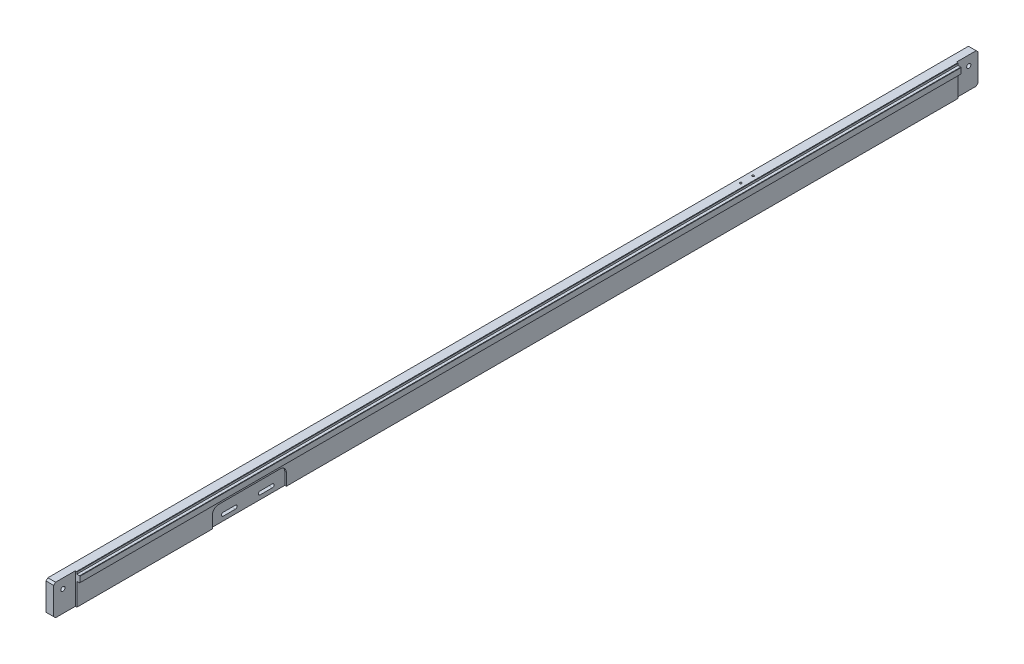
SolidWorks part; units mm, degrees
material "Al6061"
ref_plane "Front" through (0, 0, 0) normal (0, 0, 1) x (1, 0, 0)
ref_plane "Top" through (0, 0, 0) normal (0, 1, 0) x (1, 0, 0)
ref_plane "Right" through (0, 0, 0) normal (1, 0, 0) x (0, 0, -1)
sketch "草图1" plane through (0, 0, 0) normal (1, 0, 0) x (0, 0, -1)
  line L1 (-715, 25) -> (715, 25)
  line L2 (-715, 25) -> (-715, -25)
  line L3 (-715, -25) -> (715, -25)
  line L4 (715, 25) -> (715, -25)
  line L5 (-715, 25) -> (715, -25) construction
  line L6 (-715, -25) -> (715, 25) construction
  point P0 (0, 0)
  dimension "D1" = 50
  dimension "D2" = 1430
extrude "凸台-拉伸1" add sketch "草图1" along normal blind 15
sketch "草图5" plane through (15, 0, 0) normal (1, 0, 0) x (0, 0, -1)
  line L0 (-715, 25) -> (-715, -25) construction
  line L1 (-715, 21.5) -> (715, 21.5)
  line L2 (-715, 21.5) -> (-715, 11.5)
  line L3 (-715, 11.5) -> (715, 11.5)
  line L4 (715, 21.5) -> (715, 11.5)
  line L5 (715, -25) -> (715, 25) construction
  line L6 (715, 25) -> (-715, 25) construction
  dimension "D1" = 10
  dimension "D2" = 3.5
extrude "凸台-拉伸3" add sketch "草图5" along normal blind 5
hole_wizard "M6 螺纹孔2" positions "草图8" profile "草图7" tap size "M6" standard "GB"
sketch "草图8" plane through (-9.7067, -25, 33.2688) normal (0, 1, 0) x (0, 0, -1)
  line L6 (-681.7312, -17.2067) -> (-581.7312, -17.2067) construction
  line L7 (-681.7312, -24.7067) -> (-681.7312, -9.7067) construction
  line L8 (748.2688, -17.2067) -> (323.2688, -17.2067) construction
  line L9 (748.2688, -24.7067) -> (748.2688, -9.7067) construction
  point P0 (-581.7312, -17.2067)
  point P2 (-536.7312, -17.2067)
  point P29 (323.2688, -17.2067)
  point P31 (278.2688, -17.2067)
  dimension "D1" = 100
  dimension "D2" = 425
  dimension "D3" = 45
  dimension "D5" = 45
sketch "草图7" plane through (7.5, -25, 615) normal (1, 0, 0) x (0, 0, -1)
  line L0 (0, 0) -> (0, 18.5022)
  line L1 (0, 18.5022) -> (2.5, 17)
  line L2 (2.5, 17) -> (2.5, 0)
  line L5 (2.5, 0) -> (0, 0)
  line L10 (0, 18.5022) -> (-2.5, 17) construction
  line L11 (0, -6.35) -> (0, 107.95) construction
  dimension "螺纹孔钻头直径" = 5
  dimension "螺纹孔钻头深度" = 17
  dimension "导头角度" = 118
cosmetic thread "孔螺蚊线3" parameters "D1"=12, "D2"=6
cosmetic thread "孔螺蚊线4" parameters "D1"=12, "D2"=6
cosmetic thread "孔螺蚊线5" parameters "D1"=12, "D2"=6
cosmetic thread "孔螺蚊线7" parameters "D1"=12, "D2"=6
chamfer "倒角2" distance 0.5 angle 45 3 edges at (15, 25, 0) (20, 21.5, 0) (20, 11.5, 0)
sketch "草图10" plane through (0, 0, 0) normal (-1, 0, 0) x (0, 0, 1)
  line L0 (-715, 25) -> (715, 25) construction
  line L1 (-715, -25) -> (-750, -25)
  line L2 (-715, -25) -> (-715, 25)
  line L3 (-715, 25) -> (-750, 25)
  line L4 (-750, -25) -> (-750, 25)
  line L5 (715, -25) -> (750, -25)
  line L6 (715, -25) -> (715, 25)
  line L7 (715, 25) -> (750, 25)
  line L8 (750, -25) -> (750, 25)
  dimension "D1" = 35
extrude "凸台-拉伸4" add sketch "草图10" against normal blind 12.5
hole_wizard "M8 螺纹孔1" positions "草图12" profile "草图11" tap size "M8" standard "Gb" end condition through all
sketch "草图12" plane through (12.5, 0, 0) normal (1, 0, 0) x (0, 0, -1)
  line L0 (-750, 25) -> (-715, 25) construction
  line L1 (-750, -25) -> (-750, 25) construction
  line L2 (750, 25) -> (750, -25) construction
  point P0 (-735, 9.5)
  point P2 (735, 9.5)
  dimension "D1" = 15.5
  dimension "D2" = 15
  dimension "D3" = 15
sketch "草图11" plane through (12.5, 9.5, 735) normal (0, 1, 0) x (0, 0, -1)
  line L0 (0, 0) -> (0, 12.5)
  line L1 (0, 12.5) -> (3.4, 12.5)
  line L2 (3.4, 12.5) -> (3.4, 0)
  line L5 (3.4, 0) -> (0, 0)
  line L11 (0, -6.35) -> (0, 107.95) construction
  dimension "通孔螺纹孔钻头直径" = 6.8
  dimension "通孔螺纹孔钻头深度" = 12.5
cosmetic thread "孔螺蚊线1" parameters "D2"=7.6
cosmetic thread "孔螺蚊线8" parameters "D2"=7.6
chamfer "倒角3" distance 3 angle 45 4 edges at (6.25, -25, -750) (6.25, 25, -750) (6.25, -25, 750) (6.25, 25, 750)
sketch "草图13" plane through (0, 0, 0) normal (-1, 0, 0) x (0, 0, 1)
  line L0 (395, -15.5) -> (415, -15.5) construction
  line L1 (395, -12.75) -> (415, -12.75)
  line L2 (395, -18.25) -> (415, -18.25)
  line L3 (455, -15.5) -> (475, -15.5) construction
  line L4 (455, -12.75) -> (475, -12.75)
  line L5 (455, -18.25) -> (475, -18.25)
  line L7 (750, -22) -> (750, 22) construction
  arc A0 (395, -12.75) -> (395, -18.25) centre (395, -15.5) ccw
  arc A1 (415, -18.25) -> (415, -12.75) centre (415, -15.5) ccw
  arc A2 (455, -12.75) -> (455, -18.25) centre (455, -15.5) ccw
  arc A3 (475, -18.25) -> (475, -12.75) centre (475, -15.5) ccw
  circle A4 centre (735, 9.5) radius 3.4 construction
  point P2 (405, -15.5)
  point P7 (465, -15.5)
  dimension "D4" = 60
  dimension "D5" = 275
  dimension "D1" = 25
  dimension "D2" = 5.5
  dimension "D3" = 20
extrude "切除-拉伸1" cut sketch "草图13" against normal through all
sketch "草图14" plane through (15, 0, 0) normal (1, 0, 0) x (0, 0, -1)
  line L0 (-715, -25) -> (715, -25) construction
  line L1 (-495, -25) -> (-375, -25)
  line L2 (-495, -25) -> (-495, 4.5)
  line L3 (-495, 4.5) -> (-375, 4.5)
  line L4 (-375, -25) -> (-375, 4.5)
  arc A0 (-475, -12.75) -> (-475, -18.25) centre (-475, -15.5) ccw construction
  arc A1 (-395, -18.25) -> (-395, -12.75) centre (-395, -15.5) ccw construction
  arc A2 (-455, -18.25) -> (-455, -12.75) centre (-455, -15.5) ccw construction
  dimension "D1" = 20
  dimension "D2" = 20
  dimension "D3" = 20
extrude "切除-拉伸2" cut sketch "草图14" against normal blind 2.5
fillet "圆角1" radius 10 2 edges at (13.75, 4.5, 375) (13.75, 4.5, 495)
hole_wizard "M6 螺纹孔3" positions "草图16" profile "草图15" tap size "M6" standard "Iso"
sketch "草图16" plane through (0, -25, 0) normal (0, -1, 0) x (-1, 0, 0)
  line L0 (0, -747) -> (0, 747) construction
  line L1 (0, -750) -> (-12.5, -750) construction
  point P0 (-7.5, 133.512)
  point P3 (-7.5, 158.512)
  dimension "D1" = 7.5
  dimension "D2" = 25
  dimension "D3" = 883.512
sketch "草图15" plane through (7.5, -25, -133.512) normal (1, 0, 0) x (0, 0, -1)
  line L0 (0, 0) -> (0, 18.5022)
  line L1 (0, 18.5022) -> (2.5, 17)
  line L2 (2.5, 17) -> (2.5, 0)
  line L5 (2.5, 0) -> (0, 0)
  line L10 (0, 18.5022) -> (-2.5, 17) construction
  line L11 (0, -6.35) -> (0, 107.95) construction
  dimension "螺纹孔钻头直径" = 5
  dimension "螺纹孔钻头深度" = 17
  dimension "导头角度" = 118
cosmetic thread "孔螺蚊线11" parameters "D1"=12, "D2"=6
cosmetic thread "孔螺蚊线12" parameters "D1"=12, "D2"=6
hole_wizard "M6 螺纹孔5" positions "草图20" profile "草图19" tap size "M6" standard "Iso"
sketch "草图20" plane through (0, -25, 0) normal (0, -1, 0) x (-1, 0, 0)
  line L1 (0, -750) -> (-12.5, -750) construction
  point P0 (-6.25, -492.5)
  point P2 (-6.25, -387.5)
  dimension "D1" = 257.5
  dimension "D2" = 105
sketch "草图19" plane through (6.25, -25, 492.5) normal (1, 0, 0) x (0, 0, -1)
  line L0 (0, 0) -> (0, 18.5022)
  line L1 (0, 18.5022) -> (2.5, 17)
  line L2 (2.5, 17) -> (2.5, 0)
  line L5 (2.5, 0) -> (0, 0)
  line L10 (0, 18.5022) -> (-2.5, 17) construction
  line L11 (0, -6.35) -> (0, 107.95) construction
  dimension "螺纹孔钻头直径" = 5
  dimension "螺纹孔钻头深度" = 17
  dimension "导头角度" = 118
cosmetic thread "孔螺蚊线15" parameters "D1"=12, "D2"=6
cosmetic thread "孔螺蚊线16" parameters "D1"=12, "D2"=6
hole_wizard "M4 螺纹孔1" positions "草图22" profile "草图21" tap size "M4" standard "Gb"
sketch "草图22" plane through (0, 0, -750) normal (0, 0, -1) x (-1, 0, 0)
  line L0 (-12.5, 25) -> (0, 25) construction
  line L1 (0, 22) -> (0, -22) construction
  point P0 (-6.25, 15)
  point P7 (-6.25, 0)
  dimension "D1" = 10
  dimension "D2" = 6.25
  dimension "D3" = 15
sketch "草图21" plane through (6.25, 15, -750) normal (1, 0, 0) x (0, 1, 0)
  line L0 (0, 0) -> (0, 12.4914)
  line L1 (0, 12.4914) -> (1.65, 11.5)
  line L2 (1.65, 11.5) -> (1.65, 0)
  line L5 (1.65, 0) -> (0, 0)
  line L10 (0, 12.4914) -> (-1.65, 11.5) construction
  line L11 (0, -6.35) -> (0, 107.95) construction
  dimension "螺纹孔钻头直径" = 3.3
  dimension "螺纹孔钻头深度" = 11.5
  dimension "导头角度" = 118
cosmetic thread "孔螺蚊线17" parameters "D1"=8, "D2"=4
cosmetic thread "孔螺蚊线18" parameters "D1"=8, "D2"=4
hole_wizard "M4 螺纹孔2" positions "草图24" profile "草图23" tap size "M4" standard "Gb"
sketch "草图24" plane through (0, 25, 0) normal (0, 1, 0) x (1, 0, 0)
  line L0 (0, 747) -> (0, -747) construction
  line L1 (0, 750) -> (12.5, 750) construction
  point P0 (7.5, 390)
  point P2 (7.5, 370)
  dimension "D1" = 7.5
  dimension "D2" = 20
  dimension "D3" = 360
sketch "草图23" plane through (7.5, 25, -390) normal (1, 0, 0) x (0, 0, 1)
  line L0 (0, 0) -> (0, 12.4914)
  line L1 (0, 12.4914) -> (1.65, 11.5)
  line L2 (1.65, 11.5) -> (1.65, 0)
  line L5 (1.65, 0) -> (0, 0)
  line L10 (0, 12.4914) -> (-1.65, 11.5) construction
  line L11 (0, -6.35) -> (0, 107.95) construction
  dimension "螺纹孔钻头直径" = 3.3
  dimension "螺纹孔钻头深度" = 11.5
  dimension "导头角度" = 118
cosmetic thread "孔螺蚊线19" parameters "D1"=8, "D2"=4
cosmetic thread "孔螺蚊线20" parameters "D1"=8, "D2"=4
hole_wizard "M4 螺纹孔3" positions "草图26" profile "草图25" tap size "M4" standard "Gb"
sketch "草图26" plane through (0, -25, 0) normal (0, -1, 0) x (-1, 0, 0)
  line L0 (0, -747) -> (0, 747) construction
  line L1 (0, -750) -> (-12.5, -750) construction
  point P0 (-7.5, 122.012)
  point P2 (-7.5, 102.012)
  point P4 (-7.5, 82.012)
  point P6 (-7.5, 62.012)
  point P8 (-7.5, 42.012)
  dimension "D1" = 7.5
  dimension "D2" = 20
  dimension "D3" = 20
  dimension "D4" = 20
  dimension "D5" = 20
  dimension "D6" = 792.012
sketch "草图25" plane through (7.5, -25, -122.012) normal (1, 0, 0) x (0, 0, -1)
  line L0 (0, 0) -> (0, 12.4914)
  line L1 (0, 12.4914) -> (1.65, 11.5)
  line L2 (1.65, 11.5) -> (1.65, 0)
  line L5 (1.65, 0) -> (0, 0)
  line L10 (0, 12.4914) -> (-1.65, 11.5) construction
  line L11 (0, -6.35) -> (0, 107.95) construction
  dimension "螺纹孔钻头直径" = 3.3
  dimension "螺纹孔钻头深度" = 11.5
  dimension "导头角度" = 118
cosmetic thread "孔螺蚊线21" parameters "D1"=8, "D2"=4
cosmetic thread "孔螺蚊线22" parameters "D1"=8, "D2"=4
cosmetic thread "孔螺蚊线23" parameters "D1"=8, "D2"=4
cosmetic thread "孔螺蚊线24" parameters "D1"=8, "D2"=4
cosmetic thread "孔螺蚊线25" parameters "D1"=8, "D2"=4
